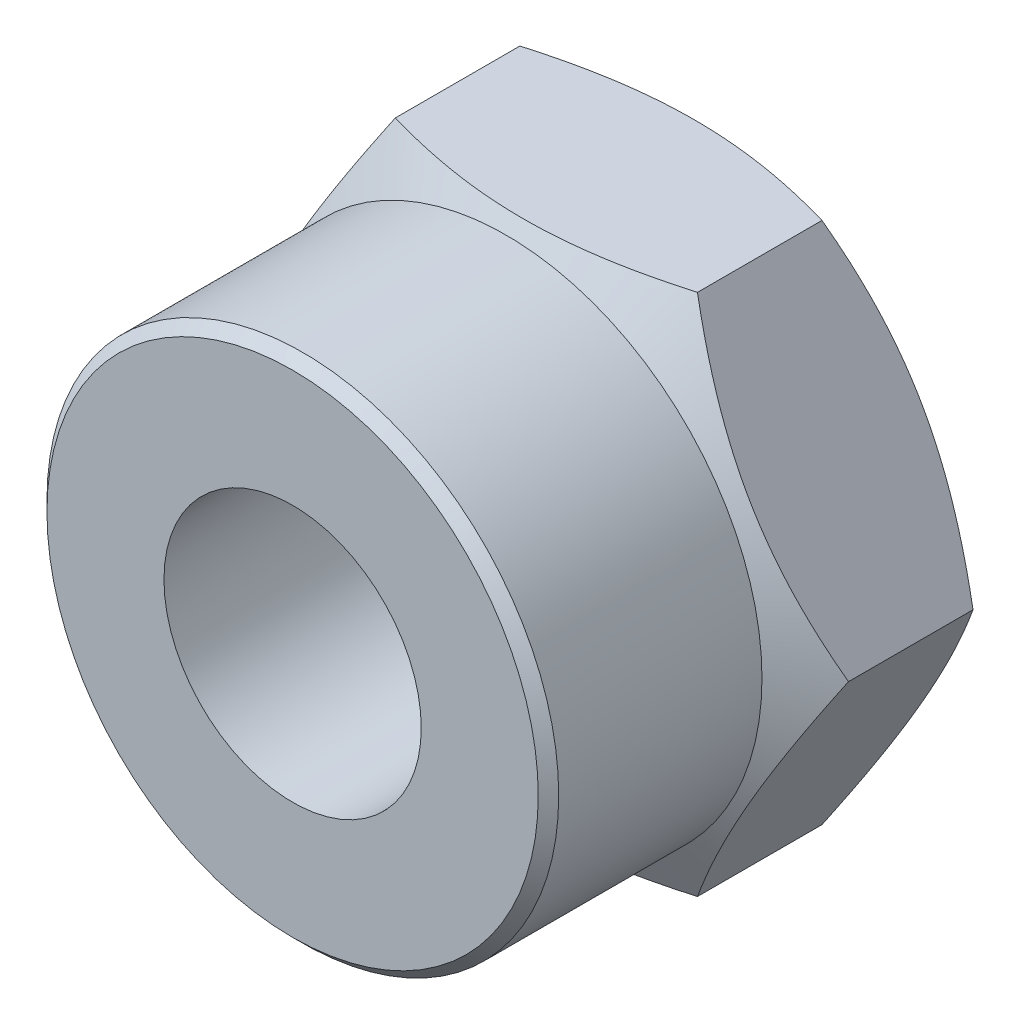
from build123d import *

# Parameters (mm, degrees)
SKETCH1_R      = 2.4585
BASENUT_DEPTH  = 3.92
EXTRUDE1_START = 4.08
SKETCH2_R      = 4.89
SKETCH2_R_2    = 2.4585
EXTRUDE1_DEPTH = 4.08
CHAMFER1_SIZE  = 0.1956


with BuildPart() as part:
    # Sketch1 → BaseNut (new body)
    with BuildSketch(Plane.XY):
        Polygon((2.886751346, -5), (5.773502692, 0), (2.886751346, 5), (-2.886751346, 5), (-5.773502692, 0), (-2.886751346, -5), align=None)
        Circle(SKETCH1_R, mode=Mode.SUBTRACT)
    extrude(amount=-BASENUT_DEPTH)

    # Sketch3 → Double-Chamfer (revolve, cut)
    with BuildSketch(Plane(origin=(0, 0, 0), x_dir=(1, 0, 0), z_dir=(0, 1, 0)), mode=Mode.PRIVATE) as double_chamfer_sk:
        Polygon((4.44, 3.92), (5.773502692, 3.92), (5.773502692, 3.150101862), align=None)
        Polygon((5.773502692, 0.769898138), (4.44, 0), (5.773502692, 0), align=None)
    revolve(double_chamfer_sk.sketch.rotate(Axis((0, 0, -16.31077227), (0, 0, 1)), 179.999999973), axis=Axis((0, 0, -16.31077227), (0, 0, 1)), mode=Mode.SUBTRACT)

    # Sketch2 → Extrude1 (add)
    with BuildSketch(Plane(origin=(20.087129569, -4.281493882, 0), x_dir=(1, 0, 0), z_dir=(0, 0, 1)).offset(EXTRUDE1_START)):
        with Locations((-20.087129569, 4.281493882)):
            Circle(SKETCH2_R)
        with Locations((-20.087129569, 4.281493882)):
            Circle(SKETCH2_R_2, mode=Mode.SUBTRACT)
    extrude(amount=-EXTRUDE1_DEPTH)

    # Sketch5 → EndChamfer (revolve, cut)
    with BuildSketch(Plane(origin=(0, 0, 0), x_dir=(1, 0, 0), z_dir=(0, 1, 0))):
        Polygon((2.4585, 3.92), (3.375, 3.92), (2.4585, 3.0035), align=None)
    revolve(axis=Axis((0, 0, -16.800797033), (0, 0, 1)), mode=Mode.SUBTRACT)

    # Chamfer1
    chamfer1_edges = [part.edges().sort_by_distance(p)[0] for p in [
        (-4.89, 0, 4.08),
    ]]
    chamfer(chamfer1_edges, length=CHAMFER1_SIZE)


solid = part.part
